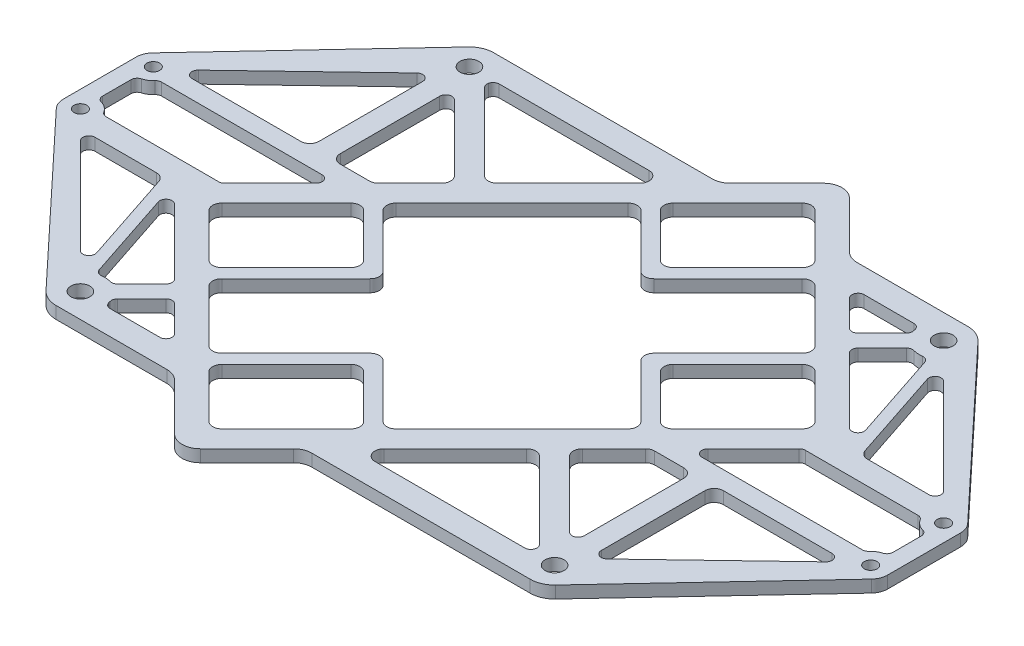
SolidWorks part; units mm, degrees
material "Thornel Mat VMA"
ref_plane "前视基准面" through (0, 0, 0) normal (0, 0, 1) x (1, 0, 0)
ref_plane "上视基准面" through (0, 0, 0) normal (0, 1, 0) x (1, 0, 0)
ref_plane "右视基准面" through (0, 0, 0) normal (1, 0, 0) x (0, 0, -1)
other "Configuration Table"
sketch "草图1" plane through (0, 0, 0) normal (0, 1, 0) x (1, 0, 0)
  line L0 (0, 0) -> (82.211, 82.211) construction
  line L1 (-65, 6) -> (65, 6) construction
  line L2 (-65, 6) -> (-65, -6) construction
  line L3 (-65, -6) -> (65, -6) construction
  line L4 (65, 6) -> (65, -6) construction
  line L5 (-65, 6) -> (65, -6) construction
  line L6 (-65, -6) -> (65, 6) construction
  line L7 (46.669, 8.8388) -> (-8.8388, -46.669)
  line L8 (46.669, 8.8388) -> (8.8388, 46.669)
  line L9 (-8.8388, -46.669) -> (-46.669, -8.8388)
  line L10 (8.8388, 46.669) -> (-46.669, -8.8388)
  line L11 (46.669, 8.8388) -> (-46.669, -8.8388) construction
  line L12 (-8.8388, -46.669) -> (8.8388, 46.669) construction
  line L13 (0, 0) -> (0, -179.5096) construction
  line L14 (0, 0) -> (80.8933, 0) construction
  line L15 (8.8388, 41.0122) -> (-41.0122, -8.8388)
  line L16 (-8.8388, -41.0122) -> (-41.0122, -8.8388)
  line L17 (41.0122, 8.8388) -> (-8.8388, -41.0122)
  line L18 (41.0122, 8.8388) -> (8.8388, 41.0122)
  line L19 (36, -29) -> (43.8666, -29) construction
  line L20 (36, -29) -> (36, -35) construction
  line L21 (-36, -29) -> (-36, -35) construction
  line L22 (-36, -29) -> (-43.8666, -29) construction
  line L23 (-67.8, 6) -> (-67.8, -6)
  line L24 (-67.0435, 7.9142) -> (-41.9192, 34.7346)
  line L25 (-65, 3.2) -> (-65, -3.2)
  line L26 (-67.0435, -7.9142) -> (-41.9192, -34.7346)
  line L27 (-62.6357, 7.5) -> (-40.75, 28.4031)
  line L28 (-63.0201, -7.9799) -> (-41.8284, -29.1716)
  line L29 (-39, 36) -> (-1.8302, 36)
  line L30 (-39, -36) -> (-19.5079, -36)
  line L31 (-35, -32) -> (-23.5079, -32)
  line L32 (-35, 32) -> (-5.8302, 32)
  line L33 (-39, 32) -> (-22.4151, 15.4151) construction
  line L34 (-35.2192, 30.6941) -> (-21.1777, 16.6525)
  line L35 (-37.6941, 28.2192) -> (-23.6525, 14.1777)
  line L36 (-39, -32) -> (-31.2539, -24.2539) construction
  line L37 (-37.4386, -28.3173) -> (-32.3146, -23.1933)
  line L38 (-35.3173, -30.4386) -> (-30.1933, -25.3146)
  line L39 (-62.6357, 7.5) -> (-30.3302, 7.5)
  line L40 (-62.6357, 4.5) -> (-33.3302, 4.5)
  line L41 (-62.3847, -5) -> (-42.8302, -5)
  line L42 (-46.669, -8.8388) -> (-62.1612, -8.8388)
  line L43 (-39, 32) -> (-39, 6) construction
  line L44 (-40.75, 28.4031) -> (-40.75, 7.5)
  line L45 (-37.25, 28.4031) -> (-37.25, 7.5)
  line L46 (67.0435, -7.9142) -> (41.9192, -34.7346)
  line L47 (62.6357, -7.5) -> (40.75, -28.4031)
  line L48 (40.75, -28.4031) -> (40.75, -7.5)
  line L49 (37.25, -28.4031) -> (37.25, -7.5)
  line L50 (37.6941, -28.2192) -> (23.6525, -14.1777)
  line L51 (35.2192, -30.6941) -> (21.1777, -16.6525)
  line L52 (35, -32) -> (5.8302, -32)
  line L53 (39, -36) -> (1.8302, -36)
  line L54 (62.6357, -7.5) -> (30.3302, -7.5)
  line L55 (67.8, -6) -> (67.8, 6)
  line L56 (62.6357, -4.5) -> (33.3302, -4.5)
  line L57 (65, -3.2) -> (65, 3.2)
  line L58 (67.0435, 7.9142) -> (41.9192, 34.7346)
  line L59 (63.0201, 7.9799) -> (41.8284, 29.1716)
  line L60 (46.669, 8.8388) -> (62.1612, 8.8388)
  line L61 (62.3847, 5) -> (42.8302, 5)
  line L62 (37.4386, 28.3173) -> (32.3146, 23.1933)
  line L63 (35.3173, 30.4386) -> (30.1933, 25.3146)
  line L64 (35, 32) -> (23.5079, 32)
  line L65 (39, 36) -> (19.5079, 36)
  line L66 (-46.669, -8.8388) -> (-39, -32) construction
  line L67 (-46.669, -8.8388) -> (-40.2573, -28.2027)
  line L68 (-41.8284, -29.1716) -> (-48.5609, -8.8388)
  line L69 (40.2573, 28.2027) -> (46.669, 8.8388)
  line L70 (41.8284, 29.1716) -> (48.5609, 8.8388)
  circle A0 centre (-65, 6) radius 1.05
  circle A1 centre (-65, -6) radius 1.05
  circle A2 centre (65, 6) radius 1.05
  circle A3 centre (65, -6) radius 1.05
  circle A4 centre (39, -32) radius 1.55
  circle A5 centre (-39, -32) radius 1.55
  circle A6 centre (39, 32) radius 1.55
  circle A7 centre (-39, 32) radius 1.55
  circle A8 centre (-65, 6) radius 2.8
  circle A9 centre (-65, -6) radius 2.8
  circle A10 centre (-39, 32) radius 4
  circle A11 centre (-39, -32) radius 4
  circle A12 centre (39, -32) radius 4
  circle A13 centre (65, -6) radius 2.8
  circle A14 centre (65, 6) radius 2.8
  circle A15 centre (39, 32) radius 4
  point P0 (0, 0)
  point P135 (0, 0)
  dimension "D3" = 2.1
  dimension "D7" = 3.1
  dimension "D11" = 3
  dimension "D14" = 8
  dimension "D1" = 12
  dimension "D2" = 130
  dimension "D4" = 45
  dimension "D5" = 78.5
  dimension "D6" = 53.5
  dimension "D8" = 39
  dimension "D10" = 3
  dimension "D12" = 6
  dimension "D13" = 32
  dimension "D15" = 2.8
  dimension "D16" = 1.75
  dimension "D17" = 1.75
  dimension "D18" = 1.5
  dimension "D19" = 1.5
  dimension "D20" = 1.5
  dimension "D21" = 1.5
  dimension "D22" = 1
  dimension "D23" = 1.75
  dimension "D24" = 1.75
  dimension "D9" = 4
  dimension "D25" = 2
extrude "凸台-拉伸1" add sketch "草图1" along normal blind 2
sketch "草图2" plane through (0, 2, 0) normal (0, 1, 0) x (1, 0, 0)
  line L0 (-3.8891, 28.2843) -> (5.3033, 19.0919)
  line L1 (8.8388, 41.0122) -> (-41.0122, -8.8388) construction
  line L2 (5.3033, 19.0919) -> (18.0312, 31.8198)
  line L3 (41.0122, 8.8388) -> (8.8388, 41.0122) construction
  line L4 (-5.4801, 26.6933) -> (5.3033, 15.9099)
  line L5 (5.3033, 15.9099) -> (19.6222, 30.2288)
  line L6 (-3.8891, 28.2843) -> (-5.4801, 26.6933)
  line L7 (18.0312, 31.8198) -> (19.6222, 30.2288)
  line L8 (0, 0) -> (-69.8555, 69.8555) construction
  line L9 (0, 0) -> (45.5957, 45.5957) construction
  line L10 (-31.8198, -18.0312) -> (-30.2288, -19.6222)
  line L11 (-15.9099, -5.3033) -> (-30.2288, -19.6222)
  line L12 (-19.0919, -5.3033) -> (-31.8198, -18.0312)
  line L13 (-28.2843, 3.8891) -> (-19.0919, -5.3033)
  line L14 (-28.2843, 3.8891) -> (-26.6933, 5.4801)
  line L15 (-26.6933, 5.4801) -> (-15.9099, -5.3033)
  line L16 (31.8198, 18.0312) -> (30.2288, 19.6222)
  line L17 (19.0919, 5.3033) -> (31.8198, 18.0312)
  line L18 (15.9099, 5.3033) -> (30.2288, 19.6222)
  line L19 (28.2843, -3.8891) -> (26.6933, -5.4801)
  line L20 (26.6933, -5.4801) -> (15.9099, 5.3033)
  line L21 (28.2843, -3.8891) -> (19.0919, 5.3033)
  line L22 (5.4801, -26.6933) -> (-5.3033, -15.9099)
  line L23 (3.8891, -28.2843) -> (5.4801, -26.6933)
  line L24 (3.8891, -28.2843) -> (-5.3033, -19.0919)
  line L25 (-5.3033, -19.0919) -> (-18.0312, -31.8198)
  line L26 (-5.3033, -15.9099) -> (-19.6222, -30.2288)
  line L27 (-18.0312, -31.8198) -> (-19.6222, -30.2288)
  dimension "D1" = 18
  dimension "D2" = 13
  dimension "D3" = 2.25
  dimension "D4" = 2.25
extrude "凸台-拉伸2" add sketch "草图2" against normal up to surface (2 mm away) up to face at (48.0452, 0, 14.4677)
fillet "1.5" radius 1.5 42 edges at (19.0919, 1, -5.3033) (41.0122, 1, -8.8388) (28.2843, 1, 3.8891) (31.8198, 1, -18.0312) (-8.8388, 1, 41.0122) (-18.0312, 1, 31.8198) (3.8891, 1, 28.2843) (-5.3033, 1, 19.0919) (5.4801, 1, 26.6933) (-5.3033, 1, 15.9099) (-19.6222, 1, 30.2288) (-30.2288, 1, 19.6222) (-15.9099, 1, 5.3033) (-26.6933, 1, -5.4801) (-5.4801, 1, -26.6933) (19.6222, 1, -30.2288) (30.2288, 1, -19.6222) (15.9099, 1, -5.3033) (26.6933, 1, 5.4801) (5.3033, 1, -15.9099) (5.3033, 1, -19.0919) (18.0312, 1, -31.8198) (-3.8891, 1, -28.2843) (8.8388, 1, -41.0122) (-19.0919, 1, 5.3033) (-31.8198, 1, 18.0312) (-41.0122, 1, 8.8388) (-28.2843, 1, -3.8891) (40.75, 1, 7.5) (48.5609, 1, -8.8388) (37.25, 1, 7.5) (30.3302, 1, 7.5) (23.6525, 1, 14.1777) (21.1777, 1, 16.6525) (5.8302, 1, 32) (-48.5609, 1, 8.8388) (-5.8302, 1, -32) (-21.1777, 1, -16.6525) (-23.6525, 1, -14.1777) (-30.3302, 1, -7.5) (-37.25, 1, -7.5) (-40.75, 1, -7.5)
fillet "1" radius 1 42 edges at (35.2192, 1, 30.6941) (35, 1, 32) (-35.2192, 1, -30.6941) (-35, 1, -32) (62.1612, 1, -8.8388) (-35, 1, 32) (-23.5079, 1, 32) (-35.3173, 1, 30.4386) (-30.1933, 1, 25.3146) (-32.3146, 1, 23.1933) (-46.669, 1, 8.8388) (-37.4386, 1, 28.3173) (-40.2573, 1, 28.2027) (-41.8284, 1, 29.1716) (-62.1612, 1, 8.8388) (32.3146, 1, -23.1933) (40.2573, 1, -28.2027) (37.4386, 1, -28.3173) (30.1933, 1, -25.3146) (35.3173, 1, -30.4386) (35, 1, -32) (23.5079, 1, -32) (46.669, 1, -8.8388) (41.8284, 1, -29.1716) (65, 1, -3.2) (62.3847, 1, -5) (42.8302, 1, -5) (33.3302, 1, 4.5) (65, 1, 3.2) (62.6357, 1, 4.5) (-62.3847, 1, 5) (-42.8302, 1, 5) (-33.3302, 1, -4.5) (-65, 1, -3.2) (-65, 1, 3.2) (-62.6357, 1, -4.5) (37.25, 1, 27.7751) (-37.25, 1, -27.7751) (-40.75, 1, -28.4031) (-62.6357, 1, -7.5) (62.6357, 1, 7.5) (40.75, 1, 28.4031)
fillet "3" radius 3 6 edges at (19.5079, 1, -36) (8.8388, 1, -46.669) (-1.8302, 1, -36) (1.8302, 1, 36) (-8.8388, 1, 46.669) (-19.5079, 1, 36)
